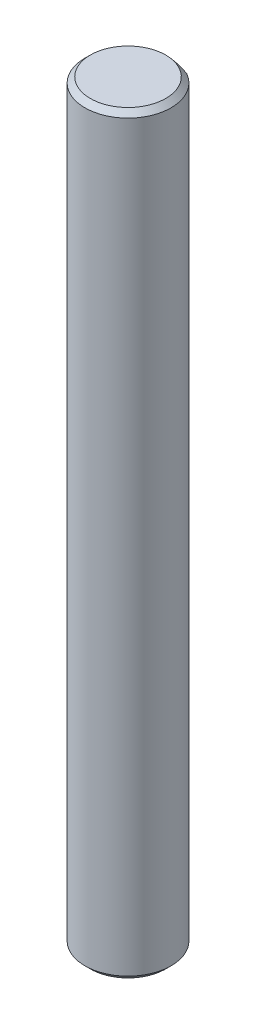
from build123d import *
from build123d.topology import SkipClean

# Parameters (mm, degrees)
SKETCH1_R           = 4
BOSS_EXTRUDE1_DEPTH = 70
CHAMFER1_SIZE       = 0.5
SKETCH2_W           = 1.564608121
SKETCH2_H           = 10
CUT_EXTRUDE1_DEPTH  = 5


with BuildPart() as part:
    # Sketch1 → Boss-Extrude1 (new body)
    with BuildSketch(Plane(origin=(0, 0, 0), x_dir=(1, 0, 0), z_dir=(0, 1, 0))):
        with Locations(Location((0, 0, 0), (0, 0, 270))):
            Circle(SKETCH1_R)
    extrude(amount=BOSS_EXTRUDE1_DEPTH)

    # Chamfer1
    chamfer1_edges = [part.edges().sort_by_distance(p)[0] for p in [
        (0, 0, -4),
        (0, 70, -4),
    ]]
    chamfer(chamfer1_edges, length=CHAMFER1_SIZE)

    # Sketch2 → Cut-Extrude1 (cut, symmetric)
    with SkipClean():  # the faces are left unmerged after this step: merging them gives an invalid solid
        with BuildSketch(Plane(origin=(0, 0, 0), x_dir=(0, 0, -1), z_dir=(1, 0, 0))):
            with Locations((4.28230406, 65)):
                Rectangle(SKETCH2_W, SKETCH2_H)
            with Locations((4.28230406, 5)):
                Rectangle(SKETCH2_W, SKETCH2_H)
        extrude(amount=CUT_EXTRUDE1_DEPTH, both=True, mode=Mode.SUBTRACT)


solid = part.part
